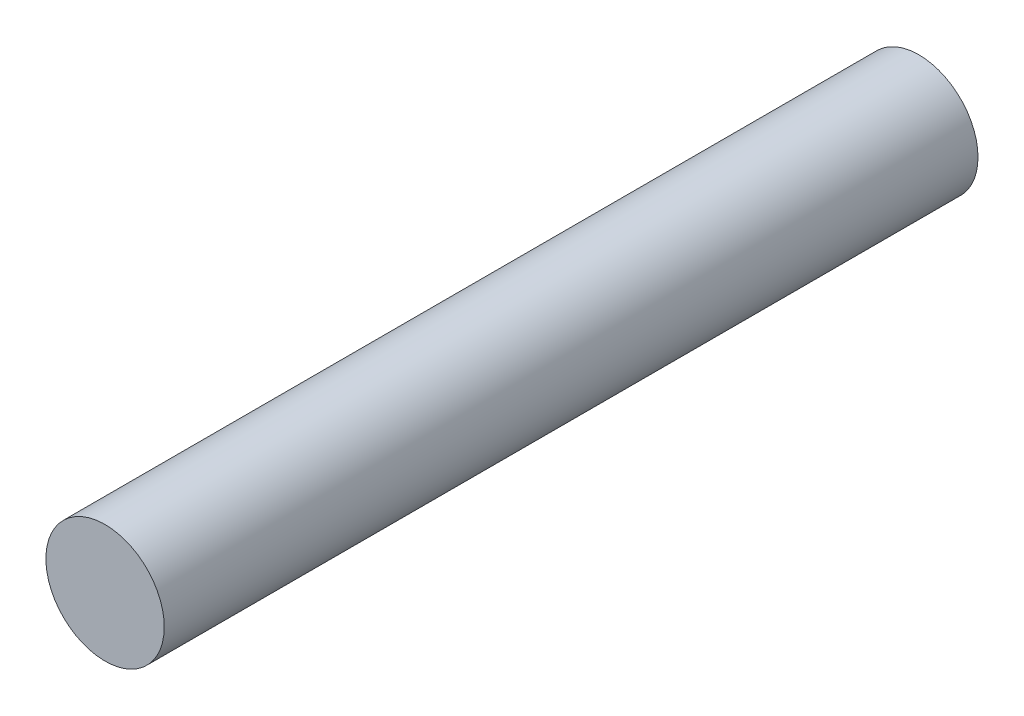
SolidWorks part; units mm, degrees
ref_plane "前视基准面" through (0, 0, 0) normal (0, 0, 1) x (1, 0, 0)
ref_plane "上视基准面" through (0, 0, 0) normal (0, 1, 0) x (1, 0, 0)
ref_plane "右视基准面" through (0, 0, 0) normal (1, 0, 0) x (0, 0, -1)
sketch "草图1" plane through (0, 0, 0) normal (0, 0, 1) x (1, 0, 0)
  circle A0 centre (0, 0) radius 4
  dimension "D1" = 8
extrude "凸台-拉伸1" add sketch "草图1" along normal mid plane 55
